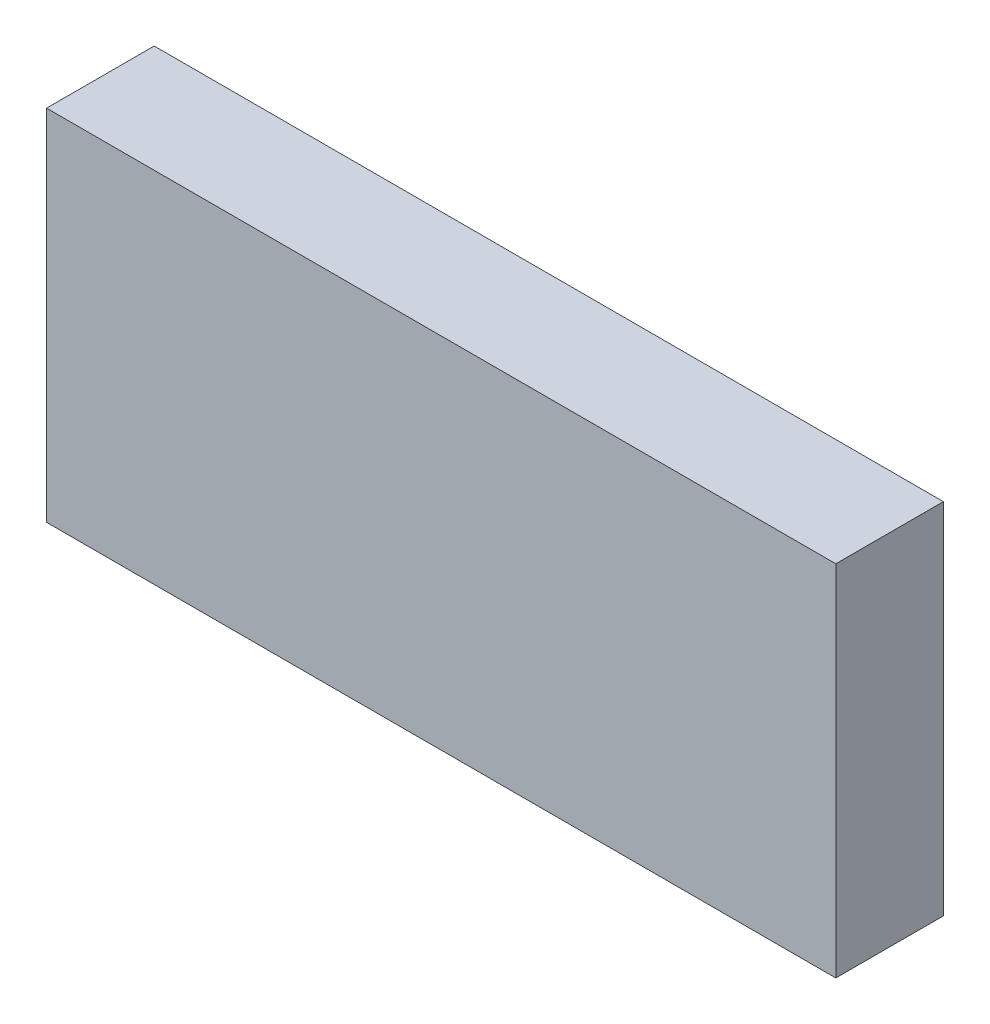
from build123d import *

# Parameters (mm, degrees)
SKETCH1_W           = 220
SKETCH1_H           = 30
BOSS_EXTRUDE1_DEPTH = 100


with BuildPart() as part:
    # Sketch1 → Boss-Extrude1 (new body)
    with BuildSketch(Plane(origin=(0, 0, 0), x_dir=(1, 0, 0), z_dir=(0, 1, 0))):
        Rectangle(SKETCH1_W, SKETCH1_H)
    extrude(amount=BOSS_EXTRUDE1_DEPTH)


solid = part.part
